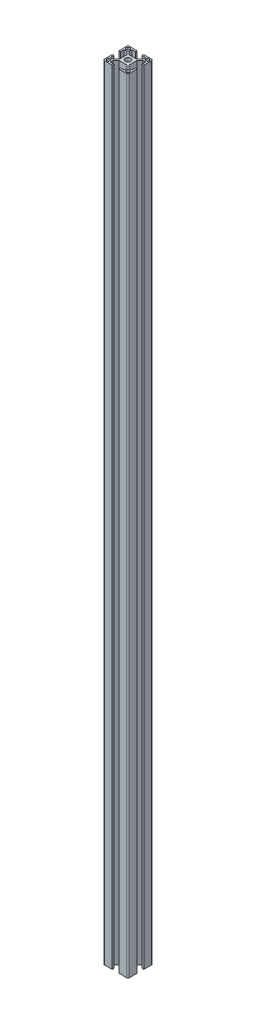
from build123d import *

# Parameters (mm, degrees)
SKETCH_1_R                = 2.1
SKETCH_1_R_2              = 3.4
EXTRUDE_1_DEPTH           = 940
HOLE_WIZARD_1_D           = 6.6
HOLE_WIZARD_1_CBORE_D     = 11
HOLE_WIZARD_1_CBORE_DEPTH = 9


with BuildPart() as part:
    # 草图1 → 拉伸1 (new body)
    with BuildSketch(Plane(origin=(0, 0, 0), x_dir=(1, 0, 0), z_dir=(0, 1, 0))):
        with BuildLine():
            Line((6.75, -28), (11, -28))
            Line((11, -28), (11, -30))
            Line((11, -30), (2, -30))
            ThreePointArc((2, -30), (0.585786438, -29.414213562), (0, -28))
            Line((0, -28), (0, -19))
            Line((0, -19), (2, -19))
            Line((2, -19), (2, -23.25))
            Line((2, -23.25), (5.335785999, -23.25))
            Line((5.335785999, -23.25), (9, -19.585785999))
            Line((9, -19.585785999), (9, -10.414214001))
            Line((9, -10.414214001), (5.335785999, -6.75))
            Line((5.335785999, -6.75), (2, -6.75))
            Line((2, -6.75), (2, -11))
            Line((2, -11), (0, -11))
            Line((0, -11), (0, -2))
            ThreePointArc((0, -2), (0.585786438, -0.585786438), (2, 0))
            Line((2, 0), (11, 0))
            Line((11, 0), (11, -2))
            Line((11, -2), (6.75, -2))
            Line((6.75, -2), (6.75, -5.335785999))
            Line((6.75, -5.335785999), (10.414214001, -9))
            Line((10.414214001, -9), (19.585785999, -9))
            Line((19.585785999, -9), (23.25, -5.335785999))
            Line((23.25, -5.335785999), (23.25, -2))
            Line((23.25, -2), (19, -2))
            Line((19, -2), (19, 0))
            Line((19, 0), (28, 0))
            ThreePointArc((28, 0), (29.414213562, -0.585786438), (30, -2))
            Line((30, -2), (30, -11))
            Line((30, -11), (28, -11))
            Line((28, -11), (28, -6.75))
            Line((28, -6.75), (24.664214001, -6.75))
            Line((24.664214001, -6.75), (21, -10.414214001))
            Line((21, -10.414214001), (21, -19.585785999))
            Line((21, -19.585785999), (24.664214001, -23.25))
            Line((24.664214001, -23.25), (28, -23.25))
            Line((28, -23.25), (28, -19))
            Line((28, -19), (30, -19))
            Line((30, -19), (30, -28))
            ThreePointArc((30, -28), (29.414213562, -29.414213562), (28, -30))
            Line((28, -30), (19, -30))
            Line((19, -30), (19, -28))
            Line((19, -28), (23.25, -28))
            Line((23.25, -28), (23.25, -24.664214001))
            Line((23.25, -24.664214001), (19.585785999, -21))
            Line((19.585785999, -21), (10.414214001, -21))
            Line((10.414214001, -21), (6.75, -24.664214001))
            Line((6.75, -24.664214001), (6.75, -28))
        make_face()
        with Locations(Location((3.375, -26.625, 0), (0, 0, 270))):
            Circle(SKETCH_1_R, mode=Mode.SUBTRACT)
        with Locations(Location((26.625, -26.625, 0), (0, 0, 270))):
            Circle(SKETCH_1_R, mode=Mode.SUBTRACT)
        with Locations(Location((15, -15, 0), (0, 0, 270))):
            Circle(SKETCH_1_R_2, mode=Mode.SUBTRACT)
        with Locations(Location((3.375, -3.375, 0), (0, 0, 270))):
            Circle(SKETCH_1_R, mode=Mode.SUBTRACT)
        with Locations(Location((26.625, -3.375, 0), (0, 0, 270))):
            Circle(SKETCH_1_R, mode=Mode.SUBTRACT)
    extrude(amount=EXTRUDE_1_DEPTH)

    # 打孔尺寸根据内六角圆柱头螺钉的类型1 (through all)
    with Locations(Plane(origin=(0, 0, 0), x_dir=(-1, 0, 0), z_dir=(0, 0, -1))):
        with Locations((-15, 895), (-15, 545), (-15, 45), (-15, 395)):
            CounterBoreHole(HOLE_WIZARD_1_D / 2, HOLE_WIZARD_1_CBORE_D / 2, HOLE_WIZARD_1_CBORE_DEPTH)


solid = part.part
